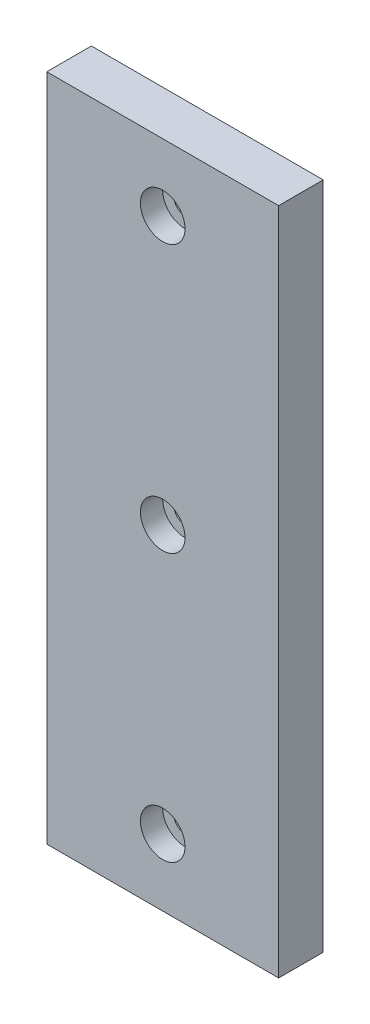
SolidWorks part; units mm, degrees
material "PA Type 6 Nylon"
ref_plane "Front Plane" through (0, 0, 0) normal (0, 0, 1) x (1, 0, 0)
ref_plane "Top Plane" through (0, 0, 0) normal (0, 1, 0) x (1, 0, 0)
ref_plane "Right Plane" through (0, 0, 0) normal (1, 0, 0) x (0, 0, -1)
sketch "Sketch1" plane through (0, 0, 0) normal (0, 0, 1) x (1, 0, 0)
  line L1 (26, -75) -> (-26, -75)
  line L2 (26, -75) -> (26, 75)
  line L3 (26, 75) -> (-26, 75)
  line L4 (-26, -75) -> (-26, 75)
  line L5 (26, -75) -> (-26, 75) construction
  line L6 (26, 75) -> (-26, -75) construction
  point P0 (0, 0)
  dimension "D1" = 150
  dimension "D2" = 52
extrude "Boss-Extrude1" add sketch "Sketch1" along normal mid plane 10
hole_wizard "Hole1" positions "Sketch2" profile "Sketch3" legacy end condition up to next
sketch "Sketch2" plane through (0, 0, 5) normal (0, 0, 1) x (1, 0, 0)
  line L0 (0, 75) -> (0, 0) construction
  line L1 (26, 75) -> (-26, 75) construction
  line L2 (0, 0) -> (-26, 0) construction
  line L3 (-26, 75) -> (-26, -75) construction
  line L4 (26, -75) -> (26, 75) construction
  point P0 (0, 60)
  point P15 (0, -60)
  point P16 (0, 0)
  dimension "D1" = 26
  dimension "D2" = 120
sketch "Sketch3" plane through (0, 60, 5) normal (1, 0, 0) x (0, -1, 0)
  line L0 (0, 0) -> (0, 10)
  line L1 (0, 10) -> (2.5, 10)
  line L2 (2.5, 10) -> (2.5, 5)
  line L3 (2.5, 5) -> (5, 5)
  line L4 (5, 5) -> (5, 0)
  line L5 (5, 0) -> (0, 0)
  line L6 (0, 110) -> (0, -10) construction
  dimension "直径" = 5
  dimension "深度" = 10
  dimension "柱坑直径" = 10
  dimension "柱坑深度" = 5
chamfer "Chamfer1" [suppressed] distance 10 angle 45
